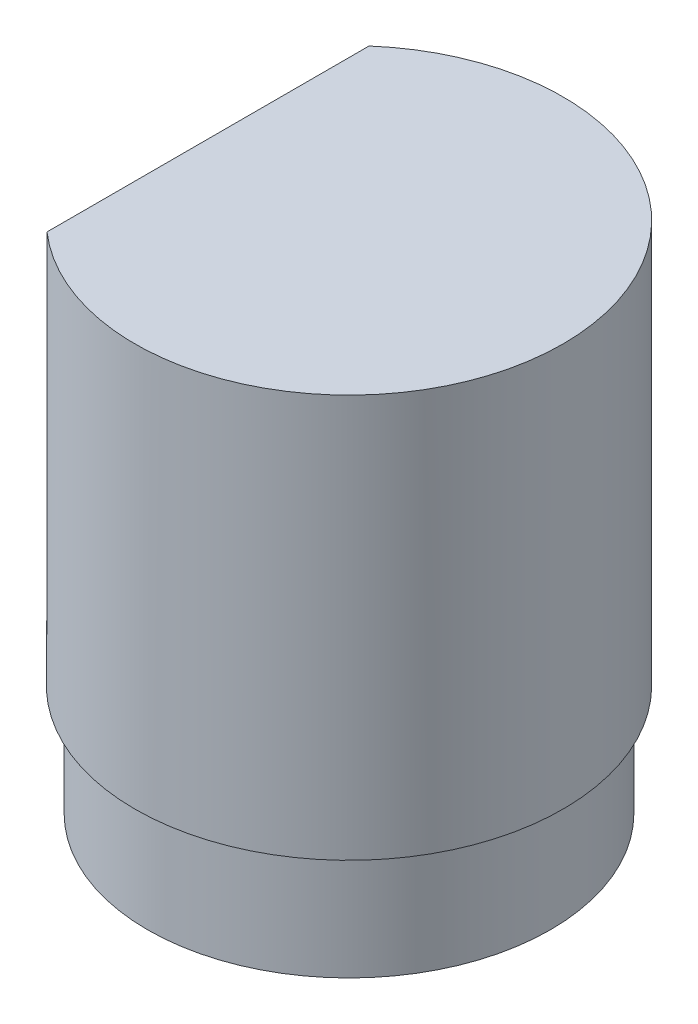
from build123d import *

# Parameters (mm, degrees)
SKETCH1_R           = 40
BOSS_EXTRUDE1_DEPTH = 22
SKETCH2_R           = 42.5
BOSS_EXTRUDE2_DEPTH = 80
CUT_EXTRUDE1_START  = -28
SKETCH3_W           = 65
SKETCH3_H           = 70
CUT_EXTRUDE1_DEPTH  = 80
SKETCH4_R           = 18.25
CUT_EXTRUDE2_DEPTH  = 90
SKETCH5_R           = 18.25
CUT_EXTRUDE3_DEPTH  = 56


with BuildPart() as part:
    # Sketch1 → Boss-Extrude1 (new body)
    with BuildSketch(Plane(origin=(0, 0, 0), x_dir=(1, 0, 0), z_dir=(0, 1, 0))):
        with Locations(Location((0, 0, 0), (0, 0, 270))):
            Circle(SKETCH1_R)
    extrude(amount=BOSS_EXTRUDE1_DEPTH)

    # Sketch2 → Boss-Extrude2 (add)
    with BuildSketch(Plane(origin=(0, 22, 0), x_dir=(1, 0, 0), z_dir=(0, 1, 0))):
        with Locations(Location((0, 0, 0), (0, 0, 270))):
            Circle(SKETCH2_R)
    extrude(amount=BOSS_EXTRUDE2_DEPTH)

    # Sketch3 → Cut-Extrude1 (cut)
    with BuildSketch(Plane(origin=(0, 0, 0), x_dir=(0, 0, -1), z_dir=(1, 0, 0)).offset(CUT_EXTRUDE1_START)):
        with Locations((0, 67)):
            Rectangle(SKETCH3_W, SKETCH3_H)
    extrude(amount=-CUT_EXTRUDE1_DEPTH, mode=Mode.SUBTRACT)

    # Sketch4 → Cut-Extrude2 (cut)
    with BuildSketch(Plane.XZ):
        with Locations(Location((0, 0, 0), (0, 0, 270))):
            Circle(SKETCH4_R)
    extrude(amount=-CUT_EXTRUDE2_DEPTH, mode=Mode.SUBTRACT)

    # Sketch5 → Cut-Extrude3 (cut)
    with BuildSketch(Plane.ZY.offset(28)):
        with Locations((0, 72)):
            Circle(SKETCH5_R)
    extrude(amount=-CUT_EXTRUDE3_DEPTH, mode=Mode.SUBTRACT)


solid = part.part
